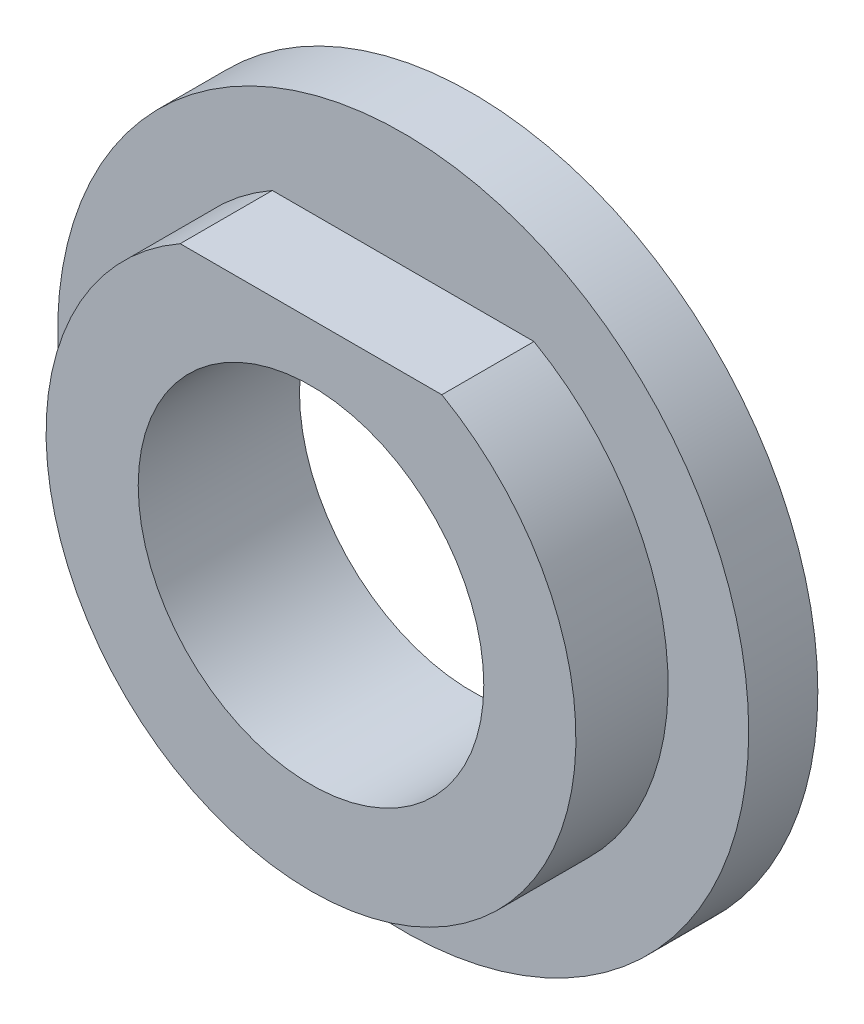
from build123d import *

# Parameters (mm, degrees)
SKETCH_1_R          = 15
SKETCH_1_R_2        = 7.5
EXTRUDE_1_DEPTH     = 7
CUT_EXTRUDE_START   = -4
SKETCH_2_R          = 15
CUT_EXTRUDE_2_DEPTH = 4


with BuildPart() as part:
    # 草图1 → 凸台-拉伸1 (new body)
    with BuildSketch(Plane.XY):
        Circle(SKETCH_1_R)
        Circle(SKETCH_1_R_2, mode=Mode.SUBTRACT)
    extrude(amount=EXTRUDE_1_DEPTH)

    # 草图2 → 切除-拉伸2 (cut)
    with BuildSketch(Plane.XY.offset(7).offset(CUT_EXTRUDE_START)):
        Circle(SKETCH_2_R)
        with BuildLine():
            Line((-5.678908346, 10), (5.678908346, 10))
            ThreePointArc((5.678908346, 10), (0, -11.5), (-5.678908346, 10))
        make_face(mode=Mode.SUBTRACT)
    extrude(amount=CUT_EXTRUDE_2_DEPTH, mode=Mode.SUBTRACT)


solid = part.part
